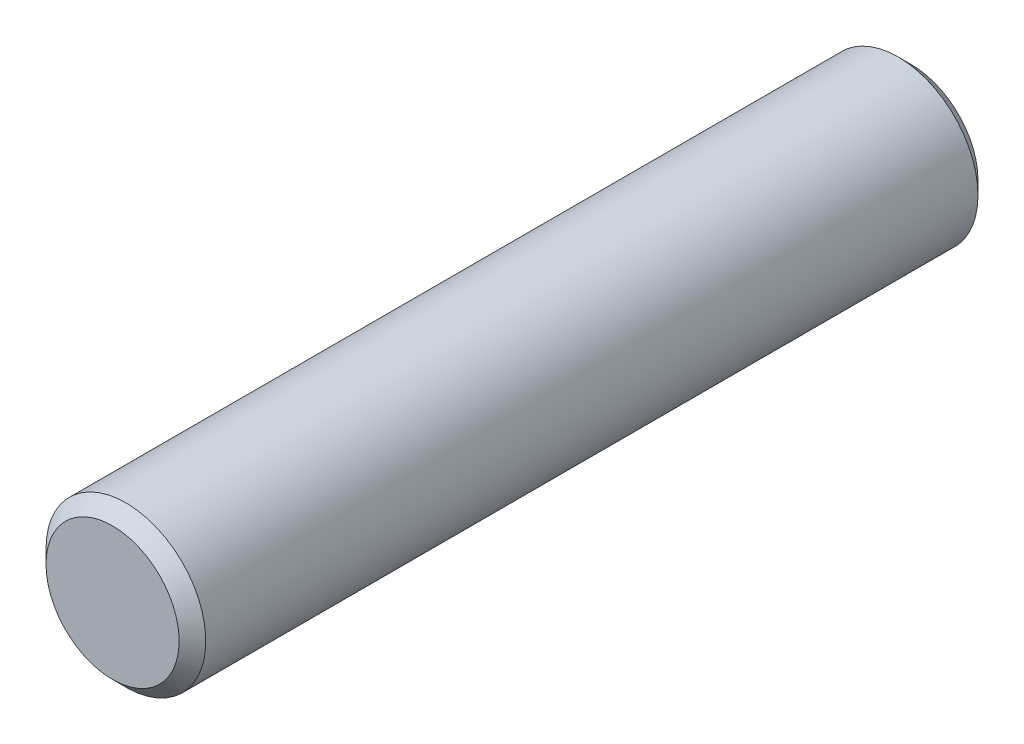
from build123d import *

# Parameters (mm, degrees)
SKETCH1_R           = 3
BOSS_EXTRUDE1_DEPTH = 30
CHAMFER1_SIZE       = 0.5


with BuildPart() as part:
    # Sketch1 → Boss-Extrude1 (new body)
    with BuildSketch(Plane.XY):
        Circle(SKETCH1_R)
    extrude(amount=BOSS_EXTRUDE1_DEPTH)

    # Chamfer1
    chamfer1_edges = [part.edges().sort_by_distance(p)[0] for p in [
        (-3, 0, 0),
        (-3, 0, 30),
    ]]
    chamfer(chamfer1_edges, length=CHAMFER1_SIZE)


solid = part.part
